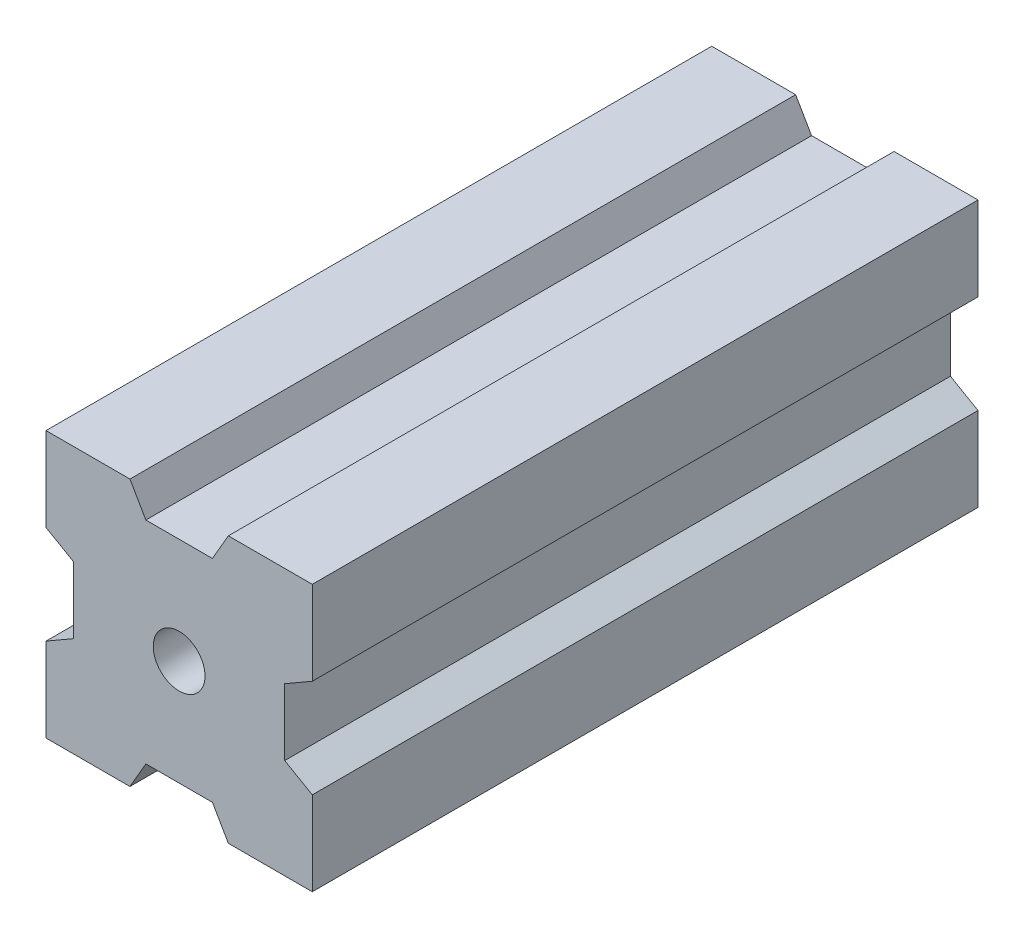
from build123d import *

# Parameters (mm, degrees)
SKETCH_1_W               = 20
SKETCH_1_H               = 20
SKETCH_1_R               = 1.94442565
EXTRUDE_1_DEPTH          = 25
CUT_EXTRUDE_1_DEPTH      = 52.961524227
PATTERN_CIRCULAR_1_COUNT = 4


with BuildPart() as part:
    # 草图1 → 凸台-拉伸1 (new, symmetric)
    with BuildSketch(Plane.XY):
        Rectangle(SKETCH_1_W, SKETCH_1_H)
        Circle(SKETCH_1_R, mode=Mode.SUBTRACT)
    extrude(amount=EXTRUDE_1_DEPTH, both=True)

    # 草图2 → 切除-拉伸1 (cut, symmetric)
    with BuildSketch(Plane.XY.offset(25)):
        Polygon((-32.933615203, 60.643738676), (-3.694439046, 10), (-2.5, 7.931170886), (2.5, 7.931170886), (3.694439046, 10), (32.933615203, 60.643738676), (32.933615203, 177.600443305), (-32.933615203, 177.600443305), align=None)
    cut_extrude_1 = extrude(amount=CUT_EXTRUDE_1_DEPTH, both=True, mode=Mode.SUBTRACT)

    # 阵列(圆周)1: 切除-拉伸1 ×4 about axis
    pattern_circular_1_axis = Axis((0, 0, 25), (0, 0, -1))
    for i in range(1, PATTERN_CIRCULAR_1_COUNT):
        add(cut_extrude_1.rotate(pattern_circular_1_axis, i * 360 / PATTERN_CIRCULAR_1_COUNT), mode=Mode.SUBTRACT)


solid = part.part
